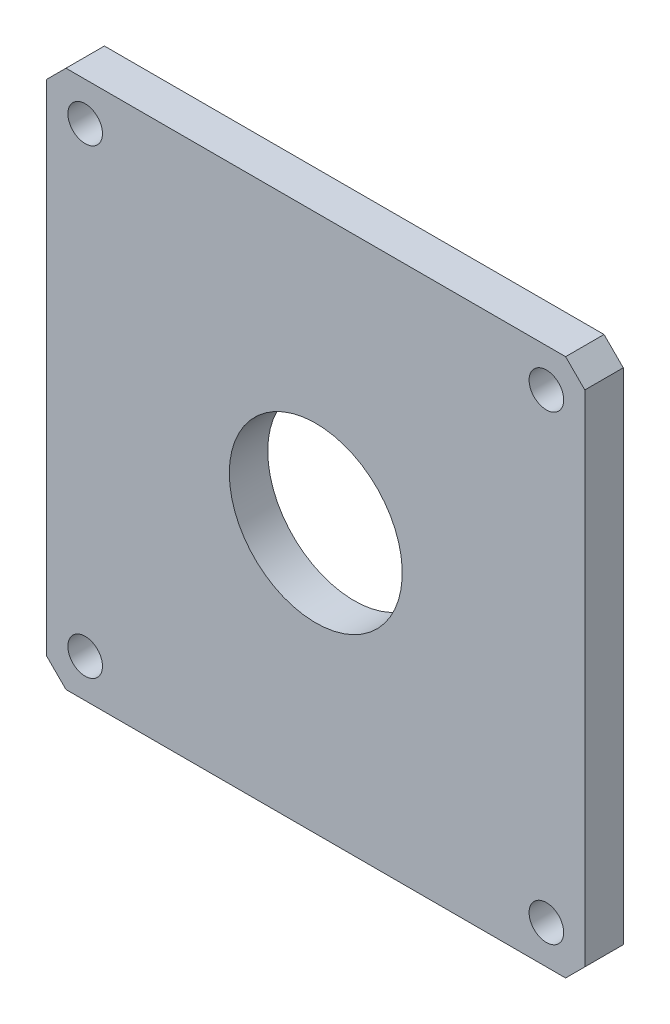
SolidWorks part; units mm, degrees
ref_plane "Front Plane" through (0, 0, 0) normal (0, 0, 1) x (1, 0, 0)
ref_plane "Top Plane" through (0, 0, 0) normal (0, 1, 0) x (1, 0, 0)
ref_plane "Right Plane" through (0, 0, 0) normal (1, 0, 0) x (0, 0, -1)
other "Configuration Table"
sketch "Sketch1" plane through (0, 0, 0) normal (0, 0, 1) x (1, 0, 0)
  line L2 (70, 70) -> (-70, 70)
  line L3 (70, 70) -> (70, -70)
  line L4 (70, -70) -> (-70, -70)
  line L5 (-70, 70) -> (-70, -70)
  line L6 (70, 70) -> (-70, -70) construction
  line L7 (70, -70) -> (-70, 70) construction
  point P2 (0, 0)
  dimension "D1" = 140
  dimension "D2" = 140
extrude "Boss-Extrude1" add sketch "Sketch1" along normal blind 10
chamfer "Chamfer1" distance 5 angle 45 4 edges at (-70, 70, 5) (70, 70, 5) (70, -70, 5) (-70, -70, 5)
hole_wizard "Ø9.0 (9) Diameter Hole1" positions "Sketch2" profile "Sketch3" hole size "Ø9.0" standard "GB"
sketch "Sketch2" plane through (0, 0, 0) normal (0, 0, -1) x (-1, 0, 0)
  line L0 (-70, -65) -> (-70, 65) construction
  line L1 (65, -70) -> (-65, -70) construction
  point P0 (-60, -60)
  dimension "D1" = 10
  dimension "D2" = 10
sketch "Sketch3" plane through (60, -60, 0) normal (1, 0, 0) x (0, 1, 0)
  line L0 (0, 0) -> (0, 22.4539)
  line L1 (0, 22.4539) -> (4.5, 19.75)
  line L2 (4.5, 19.75) -> (4.5, 0)
  line L5 (4.5, 0) -> (0, 0)
  line L10 (0, 22.4539) -> (-4.5, 19.75) construction
  line L11 (0, -6.35) -> (0, 107.95) construction
  dimension "孔直径" = 9
  dimension "孔深度" = 19.75
  dimension "导头角度" = 118
pattern_linear "LPattern1" count 2 spacing 120 along (0, 1, 0) count 2 spacing 120 along (-1, 0, 0) of "Ø9.0 (9) Diameter Hole1"
sketch "Sketch4" plane through (0, 0, 0) normal (0, 0, -1) x (-1, 0, 0)
  circle A0 centre (0, 0) radius 22.5
  dimension "D1" = 45
extrude "Cut-Extrude1" cut sketch "Sketch4" against normal blind 10
